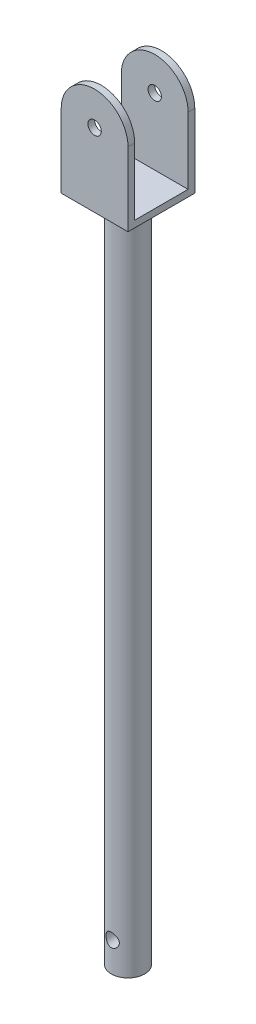
from build123d import *

# Parameters (mm, degrees)
EXTRUDE_1_DEPTH     = 10
SKETCH_2_R          = 2
CUT_EXTRUDE_1_DEPTH = 34
SKETCH_3_W          = 16
SKETCH_3_H          = 87.857567692
CUT_EXTRUDE_2_DEPTH = 17
SKETCH_5_W          = 20
SKETCH_5_H          = 20
EXTRUDE_2_DEPTH     = 2
SKETCH_6_R          = 5
EXTRUDE_3_DEPTH     = 200
SKETCH_7_R          = 2
CUT_EXTRUDE_3_DEPTH = 30.5


with BuildPart() as part:
    # 草图1 → 凸台-拉伸1 (new, symmetric)
    with BuildSketch(Plane.XY):
        with BuildLine():
            Line((-10, 20), (-10, 0))
            Line((-10, 0), (10, 0))
            Line((10, 0), (10, 20))
            ThreePointArc((10, 20), (0, 30), (-10, 20))
        make_face()
    extrude(amount=EXTRUDE_1_DEPTH, both=True)

    # 草图2 → 切除-拉伸1 (cut)
    with BuildSketch(Plane(origin=(0, 0, -10), x_dir=(-1, 0, 0), z_dir=(0, 0, -1))):
        with Locations((0, 20)):
            Circle(SKETCH_2_R)
    extrude(amount=-CUT_EXTRUDE_1_DEPTH, mode=Mode.SUBTRACT)

    # 草图3 → 切除-拉伸2 (cut, symmetric)
    with BuildSketch(Plane(origin=(0, 0, 0), x_dir=(0, 0, -1), z_dir=(1, 0, 0))):
        Rectangle(SKETCH_3_W, SKETCH_3_H)
    extrude(amount=CUT_EXTRUDE_2_DEPTH, both=True, mode=Mode.SUBTRACT)


with BuildPart() as cut_extrude_2_piece_1:
    # of the separate pieces the step leaves, piece 1, a body of its own (cut_extrude_2_pieces)
    add(part.part.solids().sort_by_distance((-10, 20, -8))[0])



with BuildPart() as cut_extrude_2_piece_2:
    # of the separate pieces the step leaves, piece 2, a body of its own (cut_extrude_2_pieces)
    add(part.part.solids().sort_by_distance((-10, 20, 10))[0])


with BuildPart() as cut_extrude_2_piece_1_1:
    add(cut_extrude_2_piece_1.part)

    add(cut_extrude_2_piece_2.part)  # 凸台-拉伸2 merges 切除-拉伸2 piece 2
    # 草图5 → 凸台-拉伸2 (add)
    with BuildSketch(Plane.XZ):
        Rectangle(SKETCH_5_W, SKETCH_5_H)
    extrude(amount=EXTRUDE_2_DEPTH)

    # 草图6 → 凸台-拉伸3 (add)
    with BuildSketch(Plane.XZ.offset(2)):
        with Locations(Location((0, 0, 0), (0, 0, 270))):
            Circle(SKETCH_6_R)
    extrude(amount=EXTRUDE_3_DEPTH)

    # 草图7 → 切除-拉伸3 (cut, symmetric)
    with BuildSketch(Plane.XY):
        with Locations(Location((0, -193.17530314, 0), (0, 0, 269.999999999))):
            Circle(SKETCH_7_R)
    extrude(amount=CUT_EXTRUDE_3_DEPTH, both=True, mode=Mode.SUBTRACT)


solid = cut_extrude_2_piece_1_1.part
